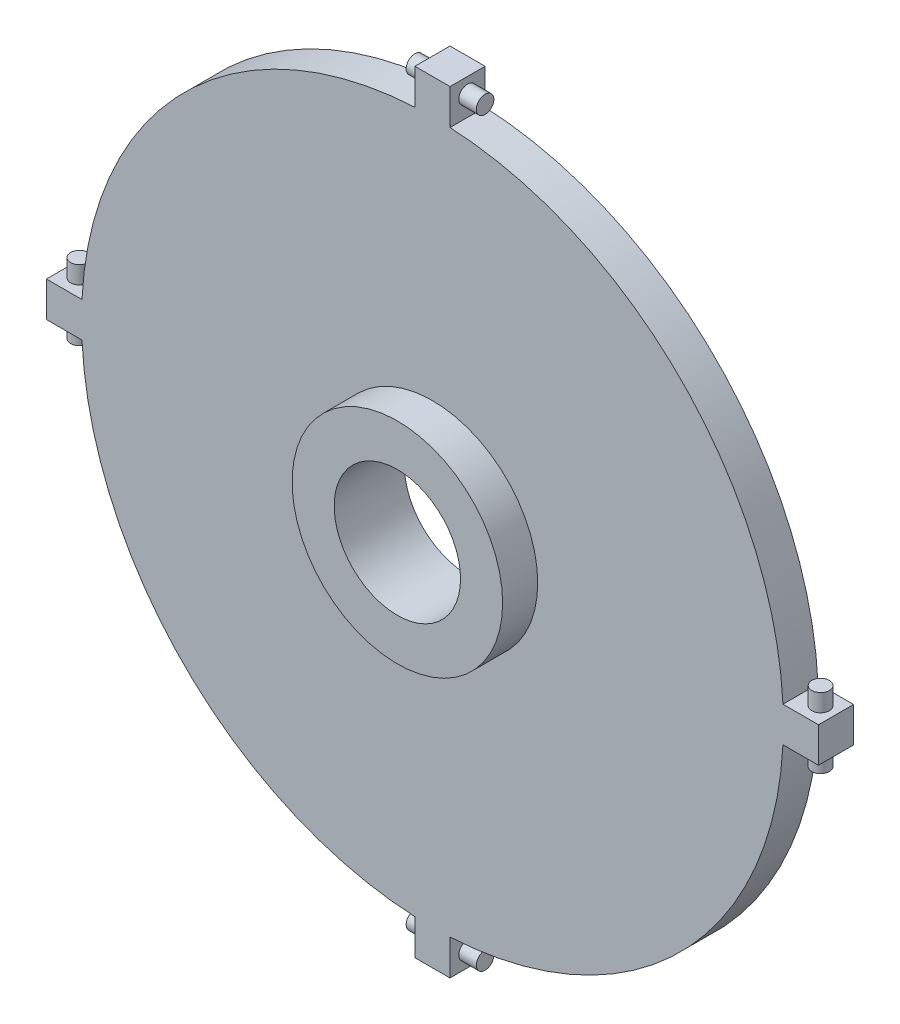
from build123d import *

# Parameters (mm, degrees)
SKETCH1_R                = 50
BOSS_EXTRUDE1_DEPTH      = 5
SKETCH2_R                = 15
BOSS_EXTRUDE2_DEPTH      = 5
SKETCH3_R                = 9
CUT_EXTRUDE1_DEPTH       = 15
BOSS_EXTRUDE3_REACH      = 118.726
BOSS_EXTRUDE3_END_RADIUS = 50
SKETCH6_R                = 1.25
BOSS_EXTRUDE4_DEPTH      = 5
CIRPATTERN3_COUNT        = 4


with BuildPart() as part:
    # Sketch1 → Boss-Extrude1 (new body)
    with BuildSketch(Plane.XY):
        Circle(SKETCH1_R)
    extrude(amount=BOSS_EXTRUDE1_DEPTH)

    # Sketch2 → Boss-Extrude2 (add)
    with BuildSketch(Plane.XY.offset(5)):
        Circle(SKETCH2_R)
    extrude(amount=BOSS_EXTRUDE2_DEPTH)

    # Sketch3 → Cut-Extrude1 (cut)
    with BuildSketch(Plane.XY.offset(10)):
        Circle(SKETCH3_R)
    extrude(amount=-CUT_EXTRUDE1_DEPTH, mode=Mode.SUBTRACT)

    # Boss-Extrude3: up to this cylinder (the profile starts outside it)
    boss_extrude3_end = Plane(origin=(0, 0, 2.5), z_dir=(0, 0, -1)) * Cylinder(BOSS_EXTRUDE3_END_RADIUS, 338.452, mode=Mode.PRIVATE)
    # Sketch4 → Boss-Extrude3 (add, up to the surface)
    with BuildSketch(Plane(origin=(0, 55, 0), x_dir=(1, 0, 0), z_dir=(0, 1, 0)), mode=Mode.PRIVATE) as boss_extrude3_sk1:
        Polygon((0, 0), (2.5, 0), (2.5, -5), (-2.5, -5), (-2.5, 0), align=None)
    boss_extrude3_tool1 = extrude(boss_extrude3_sk1.sketch, amount=-BOSS_EXTRUDE3_REACH, mode=Mode.PRIVATE) - boss_extrude3_end
    boss_extrude3 = boss_extrude3_tool1.solids().sort_by_distance((0, 55, 2.5))[0]
    add(boss_extrude3)

    # Sketch6 → Boss-Extrude4 (add, symmetric)
    with BuildSketch(Plane(origin=(0, 0, 0), x_dir=(0, 0, -1), z_dir=(1, 0, 0))):
        with Locations(Location((-2.5, 52.8, 0), (0, 0, 180))):
            Circle(SKETCH6_R)
    boss_extrude4 = extrude(amount=BOSS_EXTRUDE4_DEPTH, both=True)

    # CirPattern3: Boss-Extrude3, Boss-Extrude4 ×4 about axis
    cirpattern3_axis = Axis((0, 0, 0), (0, 0, 1))
    add([boss_extrude3.rotate(cirpattern3_axis, i * 360 / CIRPATTERN3_COUNT) for i in range(1, CIRPATTERN3_COUNT)])
    add([boss_extrude4.rotate(cirpattern3_axis, i * 360 / CIRPATTERN3_COUNT) for i in range(1, CIRPATTERN3_COUNT)])


solid = part.part
